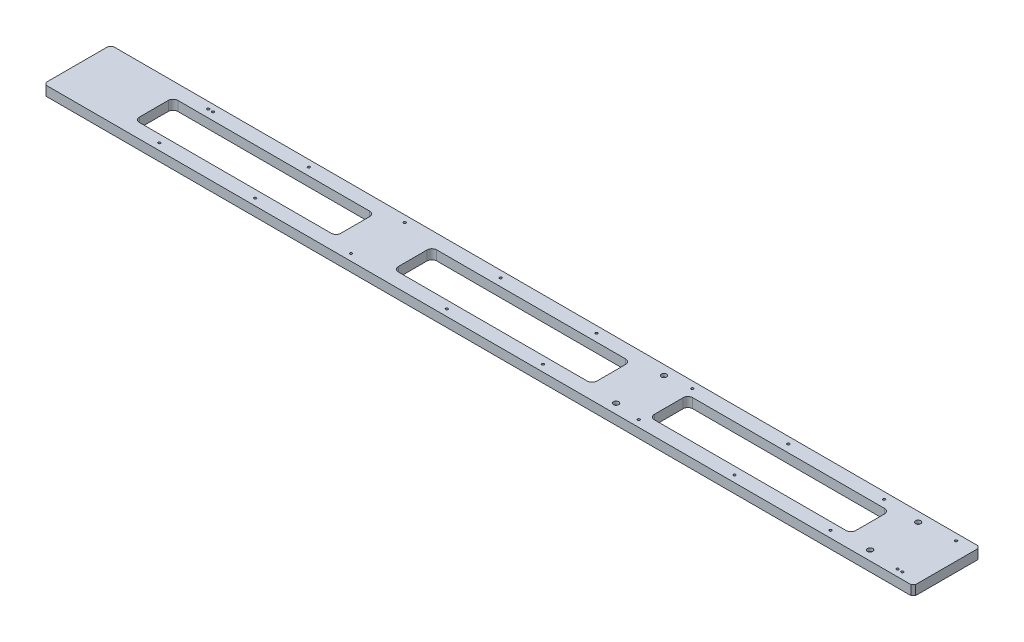
SolidWorks part; units mm, degrees
ref_plane "前视基准面" through (0, 0, 0) normal (0, 0, 1) x (1, 0, 0)
ref_plane "上视基准面" through (0, 0, 0) normal (0, 1, 0) x (1, 0, 0)
ref_plane "右视基准面" through (0, 0, 0) normal (1, 0, 0) x (0, 0, -1)
sketch "草图1" plane through (0, 0, 0) normal (0, 1, 0) x (1, 0, 0)
  line L1 (-907, -70) -> (907, -70)
  line L2 (-907, -70) -> (-907, 70)
  line L3 (-907, 70) -> (907, 70)
  line L4 (907, -70) -> (907, 70)
  line L5 (-907, -70) -> (907, 70) construction
  line L6 (-907, 70) -> (907, -70) construction
  point P0 (0, 0)
  dimension "D1" = 1814
  dimension "D2" = 140
extrude "凸台-拉伸1" add sketch "草图1" along normal blind 20
chamfer "倒角1" distance 5 angle 45 4 edges at (907, 10, 70) (-907, 10, 70) (-907, 10, -70) (907, 10, -70)
sketch "草图4" plane through (0, 20, 0) normal (0, 1, 0) x (1, 0, 0)
  point P0 (267, 50)
  point P3 (797, 50)
  point P6 (797, -50)
  point P9 (267, -50)
hole_wizard "M6 六角圆柱头螺钉的柱形沉头孔1" positions "草图4" profile "草图3" counterbore size "M6" standard "GB" end condition up to next
sketch "草图3" plane through (267, 20, -50) normal (1, 0, 0) x (0, 0, 1)
  line L0 (0, 0) -> (0, 20)
  line L1 (0, 20) -> (3.3, 20)
  line L3 (3.3, 20) -> (3.3, 6.8)
  line L4 (3.3, 6.8) -> (5.5, 6.8)
  line L5 (5.5, 6.8) -> (5.5, 0)
  line L7 (5.5, 0) -> (0, 0)
  line L11 (0, -6.35) -> (0, 107.95) construction
  dimension "通孔孔直径" = 6.6
  dimension "通孔孔深度" = 20
  dimension "柱形沉头孔直径" = 11
  dimension "柱形沉头孔深度" = 6.8
sketch "草图5" plane through (0, 0, 0) normal (0, -1, 0) x (1, 0, 0)
  line L0 (907, 65) -> (907, -65) construction
  line L1 (327, 40) -> (747, 40)
  line L2 (327, 40) -> (327, -40)
  line L3 (327, -40) -> (747, -40)
  line L4 (747, 40) -> (747, -40)
  line L5 (-902, 70) -> (902, 70) construction
  line L6 (902, -70) -> (-902, -70) construction
  line L7 (0, 0) -> (0, 413.175) construction
  line L8 (-207, 40) -> (207, 40)
  line L9 (-207, 40) -> (-207, -40)
  line L10 (-207, -40) -> (207, -40)
  line L11 (207, 40) -> (207, -40)
  line L12 (-747, 40) -> (-747, -40)
  line L13 (-327, -40) -> (-747, -40)
  line L14 (-327, 40) -> (-327, -40)
  line L15 (-327, 40) -> (-747, 40)
  dimension "D1" = 160
  dimension "D2" = 30
  dimension "D3" = 30
  dimension "D4" = 420
  dimension "D5" = 120
extrude "切除-拉伸1" cut sketch "草图5" against normal through all
fillet "圆角2" radius 10 12 edges at (-327, 10, -40) (-747, 10, 40) (-327, 10, 40) (207, 10, 40) (207, 10, -40) (-207, 10, -40) (-207, 10, 40) (747, 10, 40) (747, 10, -40) (327, 10, -40) (327, 10, 40) (-747, 10, -40)
sketch "草图8" plane through (0, 20, 0) normal (0, 1, 0) x (1, 0, 0)
  point P0 (-679.75, 56)
  point P3 (-479.75, 56)
  point P6 (-279.75, 56)
  point P9 (-79.75, 56)
  point P12 (120.25, 56)
  point P15 (320.25, 56)
  point P18 (520.25, 56)
  point P21 (720.25, 56)
  point P24 (870.25, 56)
  point P27 (870.25, -56)
  point P30 (720.25, -56)
  point P33 (520.25, -56)
  point P36 (320.25, -56)
  point P39 (120.25, -56)
  point P42 (-79.75, -56)
  point P45 (-279.75, -56)
  point P48 (-479.75, -56)
  point P51 (-679.75, -56)
hole_wizard "M6 螺纹孔1" positions "草图8" profile "草图7" tap size "M6" standard "GB" end condition through all
sketch "草图7" plane through (-679.75, 20, -56) normal (1, 0, 0) x (0, 0, 1)
  line L0 (0, 0) -> (0, 20)
  line L1 (0, 20) -> (2.5, 20)
  line L2 (2.5, 20) -> (2.5, 0)
  line L5 (2.5, 0) -> (0, 0)
  line L11 (0, -6.35) -> (0, 107.95) construction
  dimension "通孔螺纹孔钻头直径" = 5
  dimension "通孔螺纹孔钻头深度" = 20
cosmetic thread "孔螺纹线1" parameters "D2"=6
cosmetic thread "孔螺纹线2" parameters "D2"=6
cosmetic thread "孔螺纹线3" parameters "D2"=6
cosmetic thread "孔螺纹线4" parameters "D2"=6
cosmetic thread "孔螺纹线5" parameters "D2"=6
cosmetic thread "孔螺纹线6" parameters "D2"=6
cosmetic thread "孔螺纹线7" parameters "D2"=6
cosmetic thread "孔螺纹线8" parameters "D2"=6
cosmetic thread "孔螺纹线9" parameters "D2"=6
cosmetic thread "孔螺纹线10" parameters "D2"=6
cosmetic thread "孔螺纹线11" parameters "D2"=6
cosmetic thread "孔螺纹线12" parameters "D2"=6
cosmetic thread "孔螺纹线13" parameters "D2"=6
cosmetic thread "孔螺纹线14" parameters "D2"=6
cosmetic thread "孔螺纹线15" parameters "D2"=6
cosmetic thread "孔螺纹线16" parameters "D2"=6
cosmetic thread "孔螺纹线17" parameters "D2"=6
cosmetic thread "孔螺纹线18" parameters "D2"=6
sketch "草图11" plane through (0, 20, 0) normal (0, 1, 0) x (1, 0, 0)
  point P0 (-689.75, 56)
  point P3 (860.25, -56)
hole_wizard "Ø5.0mm 暗销孔1" positions "草图11" profile "草图10" hole size "Ø5.0" standard "GB"
sketch "草图10" plane through (-689.75, 20, -56) normal (1, 0, 0) x (0, 0, 1)
  line L0 (0, 0) -> (0, 16.5022)
  line L1 (0, 16.5022) -> (2.5, 15)
  line L2 (2.5, 15) -> (2.5, 0)
  line L5 (2.5, 0) -> (0, 0)
  line L10 (0, 16.5022) -> (-2.5, 15) construction
  line L11 (0, -6.35) -> (0, 107.95) construction
  dimension "孔直径" = 5
  dimension "孔深度" = 15
  dimension "导头角度" = 118
